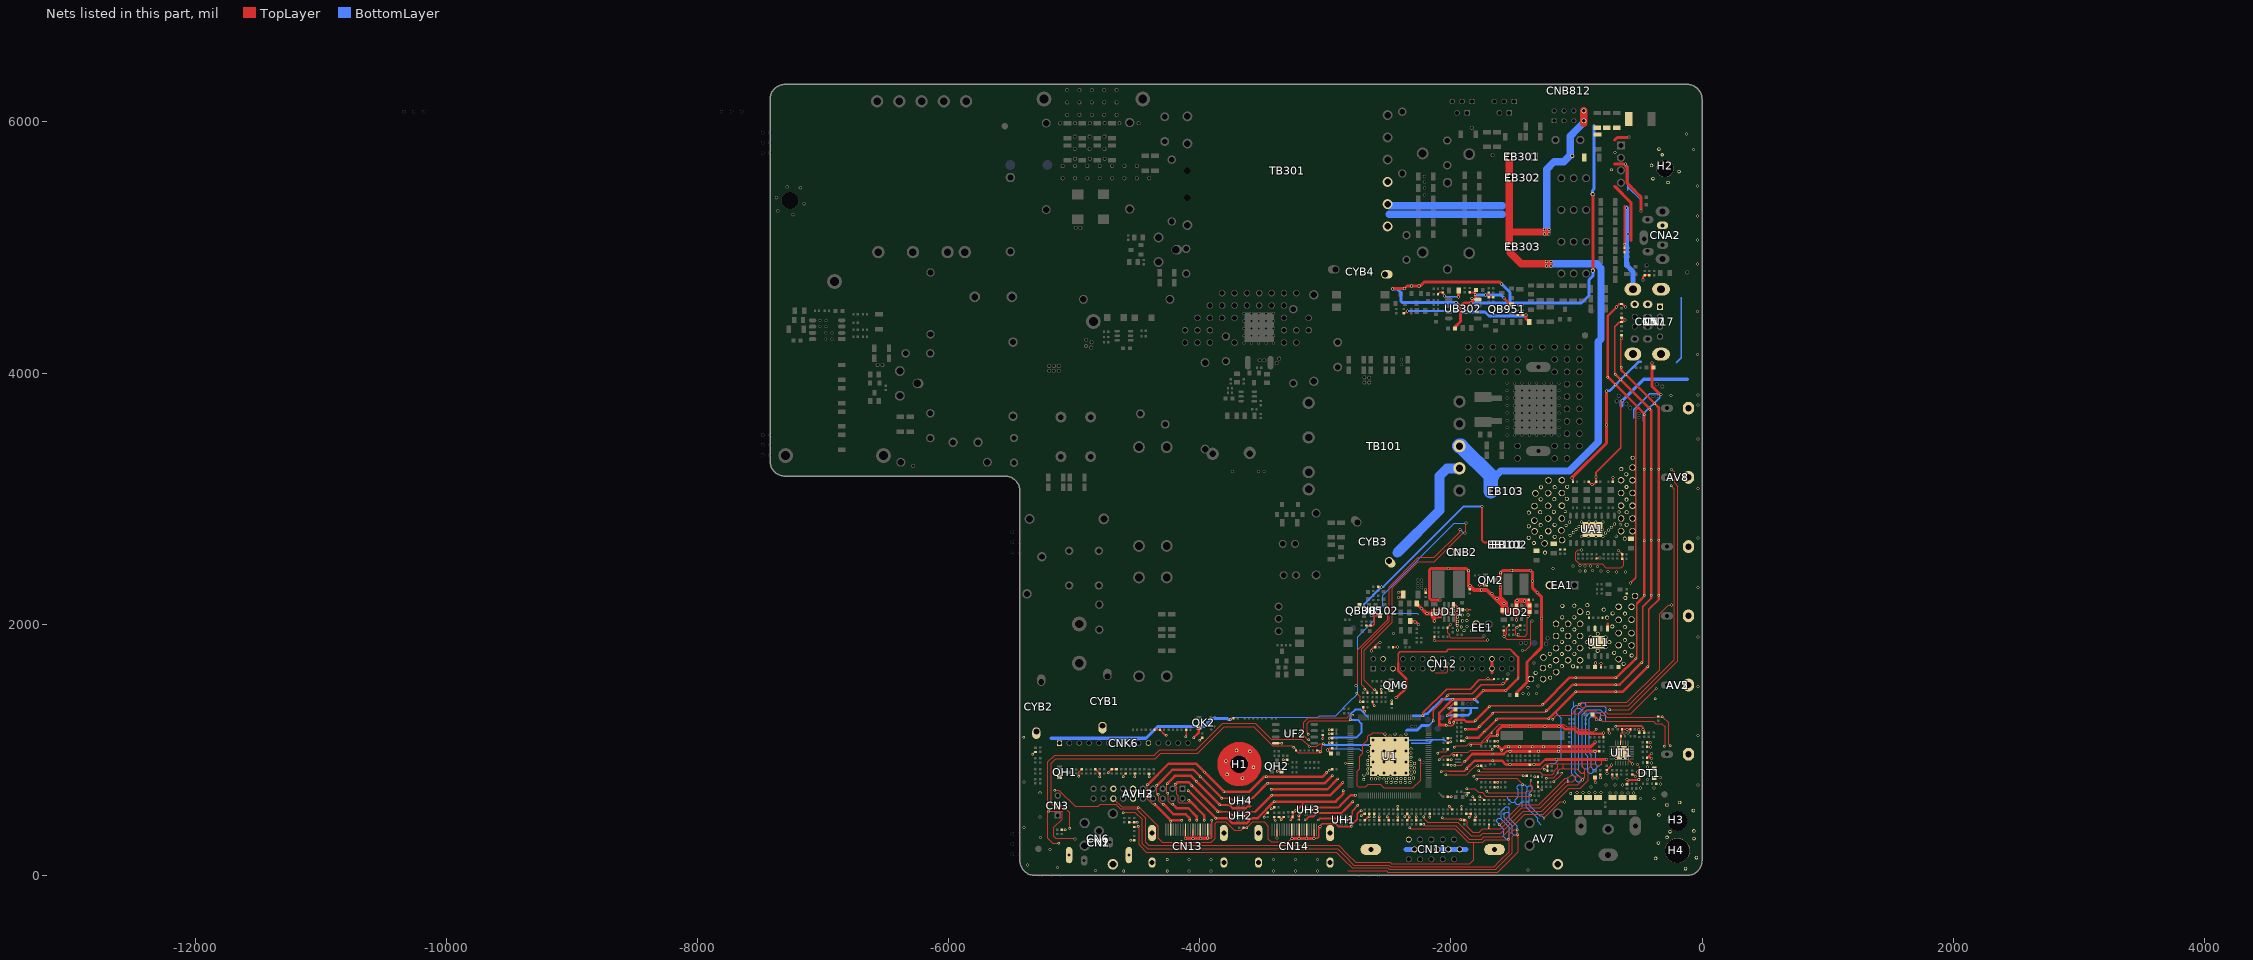
[diagram p0: the nets of this part, all layers, seen from the top]
# Altium PCB MISC84277.PcbDoc (part 8 of 15)
Units mil, origin at the board's own origin, x right, y up, seen from the top; angles counter-clockwise.
Board outline 7422.08 x 6299.21 mil, 2 copper layers (TopLayer, BottomLayer), stack 61.855 mil thick; 709 components, 395 nets, 2812 pads, 811 vias.

## Via types
v1: diameter 23.62, hole 15.75, TopLayer to BottomLayer, tented both sides, 437 vias
v2: diameter 19.68, hole 11.81, TopLayer to BottomLayer, tented both sides, 353 vias
v3: diameter 31.5, hole 23.62, TopLayer to BottomLayer, tented both sides, 16 vias
v4: diameter 31.5, hole 19.68, TopLayer to BottomLayer, tented both sides, 4 vias
v5: diameter 17.72, hole 9.84, TopLayer to BottomLayer, tented both sides, 1 vias

## Nets (pads, with @x,y where several pads share a name; then routed paths per layer and width w, separated by ;. In a path a pad name is that pad's centre, name@x,y a point inside that pad or via, vN(x,y) a via of type N, cw(c..) or ccw(c..) an arc to the next point about the centre after c; other vN are vias at no path point) (continued)
GND: AV2.2 AV2.4 AV2.6 AV5.2 AV5.4 AV5.6 AV7.1 AV8.2 AV8.4 AV8.6 AVH2.11 AVH2.12 AVH2.15 AVH2.16 AVH3.11 AVH3.12 AVH3.15 AVH3.16 C1.1 CA9.2 CA10.2 CA11.2 CA15.1 CA16.1 CA17.2 CA23.2 CA24.2 CA25.2 CA60.2 CA61.2 CB302.1 CB305.2 CB323.1 CB326.2 CB327.2 CB340.2 CB350.1 CB951.2 CD1.2 CD3.2 CD4.1 CD5.2 CD6.2 CD7.2 CD8.2 CD9.1 CD10.1 CD11.1 CD12.2 CD14.1 CD15.1 CD16.1 CD17.1 CF1.1 CF2.1 CF3.2 CF4.1 CF5.2 CF6.1 CF7.1 CF8.1 CF9.1 CF10.1 CF11.1 CF12.1 CF13.1 CF14.1 CF15.2 CF16.1 CF17.1 CF18.1 CF19.1 CF20.1 CF21.1 CF22.2 CF23.1 CF24.1 CF25.1 CF29.2 CF30.2 CF35.1 CF36.2 CF37.2 CF38.1 CF39.1 CG1.2 CG2.2 CH3.1 CH4.1 CH7.1 CH8.1 CH9.1 CH10.1 CI2.2 CI8.2 CK1.1 CK2.2 CK3.1 CK6.1 CK10.1 CL2.1 CL3.2 CL4.2 CL42.2 CL43.1 CL44.2 CM2.2 CM4.2 CM5.1 CN1.2@-4565.03,161.26 CN1.3@-5041.41,161.26 CN2.2@-4565.03,161.26 CN2.3@-5041.41,161.26 CN3.2 CN5.4 CN5.8 CN5.9 CN5.10 CN5.11 CN5.12 CN6.1 CN7.4 CN7.5 CN7.6 CN11.5 CN11.6 CN11.7 CN11.8 CN11.10 CN11.16 CN11.17 CN12.4 CN12.5 CN12.13 CN12.14 CN12.25 CN12.26 CN13.2 CN13.5 CN13.8 CN13.11 CN13.17 CN13.20 CN13.21 CN13.22 CN13.23 CN14.2 CN14.5 CN14.8 CN14.11 CN14.17 CN14.20 CN14.21 CN14.22 CN14.23 CN17.1 CNA2.1 CNB2.1 CNB812.7 CNB812.8 CNK6.1 CNK6.10 CO7.2 CO8.2 CO9.1 CO10.1 CO11.1 CT1.1 CT2.2 CT5.1 CT6.2 CT7.1 CT8.1 CT9.2 CT10.2 CT11.1 CT12.2 CT18.1 CT19.1 CT21.2 CT24.1 CT25.2 CT26.1 CT27.2 CT29.1 CT30.1 CT41.1 CT42.1 CT43.1 CT44.1 CT45.1 CT46.1 CU1.1 CV9.2 CV10.2 CYB1.1 CYB2.1 CYB3.2 CYB4.2 DB310.K DH1.A DH2.A DH3.A DH4.A DH5.A DH6.A DH7.A DH8.A DH9.A DH10.A DK1.A DT1.1 DT1.3 DU1.A DU3.A DU4.A DU7.A DU8.A EA1.2 EB101.2 EB102.2 EB103.2 EB301.2 EB302.2@-1528.48,5557.67 EB303.2@-1528.48,5005.3 EE1.2 H1.0 H1.1 H1.2 H1.3 H1.4 H1.5 H1.6 H2.0 H2.1 H2.2 H2.3 H2.4 H2.5 H2.6 H3.0 H3.1 H3.2 H3.3 H3.4 H3.5 H3.6 H4.0 H4.1 H4.2 H4.3 H4.4 H4.5 H4.6 LF6.JP_2K LT6.2 LT8.2 LT9.1 LT11.2 pad.VIA5@-534,2225 pad.VIA5@-554,2741 pad.VIA5@-554,2842.4 pad.VIA5@-554,2943.8 pad.VIA5@-554,3045.2 pad.VIA5@-554,3146.6 pad.VIA5@-554,3248 pad.VIA5@-554,3326 pad.VIA5@-562,1751 pad.VIA5@-562,1831 pad.VIA5@-562,1929 pad.VIA5@-562,2036 pad.VIA5@-562,2139 pad.VIA5@-601,2792 pad.VIA5@-601,2892 pad.VIA5@-602,2993 pad.VIA5@-602,3093 pad.VIA5@-603,3194 pad.VIA5@-611,2209 pad.VIA5@-614,2085 pad.VIA5@-615,1778 pad.VIA5@-615,1874 pad.VIA5@-615,1977 pad.VIA5@-616,2682 pad.VIA5@-625,1684 pad.VIA5@-643,3236 pad.VIA5@-645,2741 pad.VIA5@-645,2842.4 pad.VIA5@-645,2943.8 pad.VIA5@-645,3045.2 pad.VIA5@-645,3146.6 pad.VIA5@-652,2792 pad.VIA5@-660,2894 pad.VIA5@-664,1722 pad.VIA5@-664,1833 pad.VIA5@-664,1929 pad.VIA5@-664,2035 pad.VIA5@-664,2139 pad.VIA5@-684,2701 pad.VIA5@-696,2798 pad.VIA5@-701,1772 pad.VIA5@-713,2086 pad.VIA5@-715,1982 pad.VIA5@-722,2772 pad.VIA5@-738.5,1857 pad.VIA5@-746,2749 pad.VIA5@-757,2053 pad.VIA5@-770,2726 pad.VIA5@-784,2116 pad.VIA5@-831,1924.5 pad.VIA5@-831.5,1788.5 pad.VIA5@-870.08,4816.93 pad.VIA5@-872.05,5425.2 pad.VIA5@-910,2089 pad.VIA5@-913.39,2151.57 pad.VIA5@-914.5,1857.5 pad.VIA5@-971.5,1713.07 pad.VIA5@-971.5,1809.72 pad.VIA5@-971.5,1906.36 pad.VIA5@-971.5,2003 pad.VIA5@-971.5,2099.64 pad.VIA5@-979,2778 pad.VIA5@-1003,2755 pad.VIA5@-1017,1764 pad.VIA5@-1017,1858 pad.VIA5@-1017,1958 pad.VIA5@-1017,2054.64 pad.VIA5@-1017.72,2147.64 pad.VIA5@-1026,2732 pad.VIA5@-1028,1665 pad.VIA5@-1033.45,5730.08 pad.VIA5@-1051,2708 pad.VIA5@-1054.5,2812.85 pad.VIA5@-1067.25,1713.07 pad.VIA5@-1067.25,1809.72 pad.VIA5@-1067.25,1906.36 pad.VIA5@-1067.25,2003 pad.VIA5@-1075,3094 pad.VIA5@-1077,2999 pad.VIA5@-1082,2786 pad.VIA5@-1090,2896 pad.VIA5@-1112.2,2145.67 pad.VIA5@-1114,1958 pad.VIA5@-1114,2054.64 pad.VIA5@-1115,2670 pad.VIA5@-1116,1667 pad.VIA5@-1116,1763 pad.VIA5@-1116,1859 pad.VIA5@-1117,2842.4 pad.VIA5@-1117,2943.8 pad.VIA5@-1117,3045.2 pad.VIA5@-1117,3146.6 pad.VIA5@-1121,2747 pad.VIA5@-1162,1619 pad.VIA5@-1163,1713.07 pad.VIA5@-1163,1809.72 pad.VIA5@-1163,1906.36 pad.VIA5@-1163,2003 pad.VIA5@-1174,3092 pad.VIA5@-1175,2696 pad.VIA5@-1175,2791 pad.VIA5@-1177,2996 pad.VIA5@-1181,2894 pad.VIA5@-1204.72,4852.36 pad.VIA5@-1204.72,4887.8 pad.VIA5@-1210,1574 pad.VIA5@-1211,1667 pad.VIA5@-1213,1764 pad.VIA5@-1220.47,5108.27 pad.VIA5@-1220.47,5143.7 pad.VIA5@-1223.2,3145.2 pad.VIA5@-1225,2741 pad.VIA5@-1226,2841 pad.VIA5@-1226,2942.4 pad.VIA5@-1226,3043.8 pad.VIA5@-1240.16,4852.36 pad.VIA5@-1240.16,4887.8 pad.VIA5@-1251,2571 pad.VIA5@-1254,2644 pad.VIA5@-1255.91,5108.27 pad.VIA5@-1255.91,5143.7 pad.VIA5@-1264,1736 pad.VIA5@-1266,1563 pad.VIA5@-1267,1651 pad.VIA5@-1282,2694 pad.VIA5@-1283,3090.6 pad.VIA5@-1286,2790 pad.VIA5@-1286,2994.6 pad.VIA5@-1290,2892.6 pad.VIA5@-1326,1612 pad.VIA5@-1327.5,3042.5 pad.VIA5@-1334,2740 pad.VIA5@-1335,2941 pad.VIA5@-1336,2825 pad.VIA5@-1339,2647 pad.VIA5@-1363,1564 pad.VIA5@-1379.3,2889 pad.VIA5@-1380,2780 pad.VIA5@-1381,2687 pad.VIA5@-1596,4709 pad.VIA5@-1832.68,4592.52 pad.VIA5@-1836.61,1948.82 pad.VIA5@-1863,2074 pad.VIA5@-1874,2030 pad.VIA5@-1879.92,4487.1 pad.VIA5@-1895.67,1948.82 pad.VIA5@-1910,2027 pad.VIA5@-1912,2074 pad.VIA5@-1923,4495.5 pad.VIA5@-1929.13,4535.43 pad.VIA5@-1948,2022 pad.VIA5@-1948,2058 pad.VIA5@-1948.82,1952.76 pad.VIA5@-1950,1991 pad.VIA5@-1958.5,4561.5 pad.VIA5@-1980,2109 pad.VIA5@-2002,2087 pad.VIA5@-2030,2110 pad.VIA5@-2087.7,2097.06 pad.VIA5@-2253.94,4693.81 pad.VIA5@-2290.9,823 pad.VIA5@-2290.9,856.8 pad.VIA5@-2290.9,890.6 pad.VIA5@-2297.6,775.2 pad.VIA5@-2314.96,4693.81 pad.VIA5@-2319.2,805.4 pad.VIA5@-2319.2,839.2 pad.VIA5@-2319.2,873 pad.VIA5@-2319.2,906.8 pad.VIA5@-2319.2,940.6 pad.VIA5@-2319.2,974.4 pad.VIA5@-2319.2,1008.2 pad.VIA5@-2327.2,741 pad.VIA5@-2330.3,770.9 pad.VIA5@-2358.3,1124.32 pad.VIA5@-2364.1,770.9 pad.VIA5@-2364.4,741 pad.VIA5@-2370.87,4674 pad.VIA5@-2397.9,770.9 pad.VIA5@-2401.6,741 pad.VIA5@-2431.7,770.9 pad.VIA5@-2438.8,741 pad.VIA5@-2445,1124 pad.VIA5@-2465.5,769.2 pad.VIA5@-2466.54,4671.26 pad.VIA5@-2476,741 pad.VIA5@-2499.3,769.2 pad.VIA5@-2513.2,741 pad.VIA5@-2525.21,1124.32 pad.VIA5@-2533.1,769.2 pad.VIA5@-2566.9,769.2 pad.VIA5@-2600.7,769.2 pad.VIA5@-2634.5,769.2 pad.VIA5@-2635.5,864.3 pad.VIA5@-2648.2,948.3 pad.VIA5@-2662.7,814 pad.VIA5@-2662.7,847.8 pad.VIA5@-2662.7,881.6 pad.VIA5@-2662.7,915.4 pad.VIA5@-2693.4,797.4 pad.VIA5@-2694.55,765.25 QB305.E QB951.E QH1.E QH2.E QK2.E QM2.E QM6.E RA1.1 RA7.JP_2K RA9.1 RA11.JP_2K RA14.1 RB134.2 RB337.1 RB338.1 RB339.1 RB340.1 RB341.1 RB345.2 RB352.2 RB355.2 RB357.1 RB364.1 RB385.1 RB951.1 RD7.1 RD16.1 RF12.2 RF13.2 RF14.1 RF15.1 RF16.2 RF18.2 RF19.2 RH55.2 RI5.1 RI7.2 RI9.1 RI11.2 RI13.1 RI15.1 RI17.1 RI18.1 RM6.2 RM10.2 RO3.1 RO7.1 RO10.2 RO12.2 RV2.1 RV4.1 RV5.1 RV8.2 RV11.1 RV13.2 RV14.2 TB101.8@-1932.31,3241.33 TB101.9@-1932.31,3418.5 TB301.1 TB301.2@-2504.74,5345.75 TB301.3@-2504.74,5522.92 U1.116 U1.129 UA1.EPAD@-874.02,2754.94 UB102.A UB302.4 UD2.2 UD11.1 UF2.4 UH1.GND UH2.GND UH3.GND UH4.GND UL1.1 UL1.3 UL1.EPAD UT1.10 UT1.25 | length 142392
  TopLayer w4: v2(-5203.6,509.3) -5202.69,510.21 -5100.22,510.21 -5096.94,506.94 ; -3575,1210.16 -3558.36,1210.16 -3431.01,1082.81 -3334.78,1082.81
  TopLayer w5: v2(-4417.02,720.92) -4418.8,719.13 -4418.8,609.76 -4376.84,567.8 v2(-4359.93,567.8) ; v2(-4342.78,716.45) -4341.54,715.21 -4341.54,641.89 -4328.4,628.76 -4328.4,594.96 -4301.22,567.78 ; v2(-4260.82,729.12) -4262.3,727.64 -4262.3,659.1 -4249.9,646.7 -4249.9,590.49 -4226.31,566.9 v2(-4215.7,566.9) ; CN13.17@-4232.29,364.62 -4232.29,429.51 v2(-4232.1,429.7) ; v2(-4195.46,725.18) -4195.46,714.57 -4184.06,703.16 -4184.06,645.06 -4171.7,632.7 -4171.7,587 -4162.1,577.4 -4075.03,577.4 -4069.75,582.67 ; -3065.26,1031.19 -3064.24,1031.19 -3057.09,1038.34 ; UT1.25@-639.4,975.31 -574.17,910.09
  TopLayer w6: AVH2.16@-4689,610.96 -4623.14,545.1 -4518,545.1 ; v2(-4490.6,538) -4497.7,545.1 -4518,545.1 ; v2(-4146.1,273.5) -4136.1,263.5 -4127.4,263.5 ; CH10.1@-3652.97,378.1 -3670.81,360.26 -3727.16,360.26 -3792.95,426.05 -3866.44,426.05 -3877,415.5 -3877,294.47 -3907.97,263.5 -4127.4,263.5 ; v2@-3628.2,378.1 -3624.56,378.1 -3576.61,426.05 -3488.61,426.05 -3453.5,390.94 -3453.5,286.94 -3432.25,265.69 -3297.25,265.69 v1@-3267.72,295.22 ; v2(-3137,1123) -3137,1129 -3146,1138 -3146,1211.56 -3124.56,1233 -2809,1233 v2(-2801,1241) ; v2(-3132,1080) -3141,1080 -3172,1111 -3172,1219 -3136,1255 -2893,1255 ; -2880,1255 -2893,1255 ; -2852.31,123.69 -2787.68,59.06 -2503.83,59.06 -2493.14,48.38 -1642.35,48.38 -1599.23,91.5 ; -2847.42,155.58 -2772.91,81.06 -2494.72,81.06 -2484.03,70.38 -1657.12,70.38 -1610,117.5 ; v2(-2839.93,893.65) -2837.83,891.56 U1.116@-2800.46,891.56 ; -2824.54,169.46 -2760.14,105.06 -2484.77,105.06 -2474.09,94.38 -1849.62,94.38 -1818.35,125.65 -1818.35,180.15 ; v2(-2783,1277) -2790.16,1269.84 -2812.95,1269.84 -2827.79,1255 -2893,1255 ; v1(-2755.9,1513.78) -2751.97,1513.78 -2741,1524.75 -2741,1549.21 ; -2741,1553.15 -2741,1549.21 ; -2712.27,1776 -2712.27,1802.96 ; CG1.2@-2665.27,1454 -2665.27,1469.27 -2712.27,1516.27 -2712.27,1802.96 ; -2664.14,718.86 -2659.26,723.74 ; -2661.98,1087.8 -2661.98,1081.2 ; -2641.3,1119.5 -2650.57,1119.5 ; v3(-2620.6,1077.82) U1.129@-2489.44,946.68 -2489.44,1075.87 -2547.57,1134 -2550.4,1134 ; v2@-2613.58,1478.58 -2690.27,1555.27 -2690.27,1793.84 -2468,2016.11 -2468,2291.37 -2260.37,2499 -2133.27,2499 -1905.9,2726.37 v1(-1889.76,2726.37) -1881.89,2734.24 v1(-1881.89,2807.09) ; v2(-2606,1480) -2600,1480 -2591.27,1471.27 CG2.2@-2591.27,1454 ; CG2.2@-2593,1454 CG2.2@-2591.27,1454 ; CG2.2@-2591.27,1456.27 CG2.2@-2591.27,1454 ; -2571,1134 -2550.4,1134 ; v2@-2522,2084 -2521,2085 -2506.26,2085 -2501.97,2080.71 -2501.97,2034.86 -2741,1795.83 -2741,1549.21 ; v2(-2248.34,920.93) -2241.5,914.09 -2241.5,888.5 ; -2241.5,902.3 -2241.5,888.5 ; v2(-2105,973) v2@-2105,972.89 ; v2@-2100.11,968 v2@-2105,972.89 ; v2@-2092.05,922 v2(-2093,922) -2062,953 -2009,953 -1982,980 -1861.04,980 -1843.54,997.5 -1676.57,997.5 v2(-1669.72,1004.34) ; CF20.1@-2025,1006 -2025,1000 -2039,986 -2091.89,986 v2@-2105,972.89 ; v2(-1972,1022) -1963.5,1030.5 -1876.19,1030.5 -1850.19,1056.5 -1763.71,1056.5 -1691.41,1128.81 ; v1(-1929.13,2755.91) -1929.13,2734.25 -2131.89,2531.49 -2258.99,2531.49 -2490,2300.48 -2490,2236.22 -2490,2025.23 -2712.27,1802.96 ; v2(-1844.2,1037.4) -1836.96,1044.64 -1759.91,1044.64 -1740.86,1063.7 ; v2(-1713.1,1066.9) -1716.3,1063.7 -1740.86,1063.7 ; v2(-1673.1,1134.8) -1673.1,1147.11 ; -1668.6,1151.61 -1668.6,1139.3 -1679.09,1128.81 -1691.41,1128.81 ; v2(-1630,1114) -1674,1114 -1724.3,1063.7 -1740.86,1063.7 ; v2(-841.4,1163.9) -861.11,1144.19 -891.39,1144.19 -911.4,1164.2 -991.09,1164.2 -1008.99,1182.1 -1077.06,1182.1 -1100.01,1205.06 -1615.15,1205.06 -1691.41,1128.81 ; -4518,545.1 -4487.93,545.1 -4332.1,389.27 -4332.1,295.57 -4299.33,262.8 -4128.1,262.8 -4127.4,263.5 ; -2661.98,1081.2 -2702.06,1041.12 -2702.06,973.5 -2726.84,948.71 -2726.84,848.75 -2745.5,830.09 -2745.5,710.4 -2739.1,704 -2679,704 -2659.26,723.74 ; -2661.98,1081.2 -2661.98,1108.09 -2650.57,1119.5 ; -2659.26,723.74 -2561.54,723.74 -2533.63,695.83 -2304.46,695.83 -2241.5,758.78 -2241.5,888.5 ; -2650.57,1119.5 -2637.56,1119.5 -2623.06,1134 -2550.4,1134
  TopLayer w7: v1(-2131.89,1872.04) -2131.73,1872.2 RD16.1@-2131.73,1900 v1@-2131.73,1877.8 ; v2(-2078.9,827) -2076.59,824.7 v2@-2076.59,824.3 ; v2@-2078.86,829.69 -2075.31,833.24 -2017.24,833.24 -2014,830 ; v2(-2042.7,802.9) -2041.6,801.8 -1874.6,801.8 -1837.1,839.3
  TopLayer w8: v2(-5332,963.8) -5312.9,982.9 DK1.A@-5308.96,982.9 ; -5209.5,316.2 -5209.5,570.4 ; v2(-5157,679.4) -5122.8,679.4 -4993.36,549.96 -4807.52,549.96 -4791.99,565.5 -4667.9,565.5 -4632.9,530.5 -4506,530.5 -4431.5,456 -4431.5,263.7 -4406.3,238.5 -4257.2,238.5 ; v2(-5123.3,256.5) -5171.2,256.5 -5209.5,294.8 -5209.5,570.4 ; v2@-5116.3,812.98 v2(-5115.1,814.18) ; CO7.2@-5098.6,363.53 -5073.27,363.53 v2(-5072.9,363.9) ; -5096.94,506.94 -5096.94,448.3 -5162.4,382.84 -5162.4,309.9 -5146.7,294.2 -5000.2,294.2 v1(-4994.9,288.9) ; v2(-5035.9,376.9) -5035.9,496.9 -5095.36,556.36 CN3.2@-5131.53,556.36 -5165.26,556.36 -5183.5,574.6 -5183.5,892.55 -5146.2,929.84 -4353.23,929.84 -4309.87,973.2 -4017.27,973.2 -3806.32,1184.16 -3571.95,1184.16 -3418.4,1030.6 -3262.9,1030.6 v2(-3253.8,1021.5) v2@-3260.22,1021.5 ; v2(-4609.1,498.6) -4603.2,504.5 -4516.77,504.5 -4457.5,445.23 -4457.5,296.2 ; RO7.1@-4563.06,422.97 -4497.67,422.97 v2(-4497.2,422.5) ; v2(-4548.6,279.5) -4548.27,279.17 CO11.1@-4522.9,279.17 ; RO3.1@-4522.89,386.23 -4494.67,386.23 v2(-4489.4,391.5) -4483.5,385.6 -4483.5,242.16 -4425.84,184.5 -2913.12,184.5 -2852.31,123.69 ; -4457.5,317.2 -4457.5,296.2 ; -4301.5,210.5 -4290.8,210.5 ; -4269.5,238.5 -4257.2,238.5 ; v1@-4114.18,306.8 -4113.79,306.41 -3910.19,306.41 -3900,316.6 ; v1@-3936.33,295.18 -3908.82,295.18 -3900,304 -3900,316.6 ; -3910.46,303.07 -3903.21,310.32 -3903.21,423.89 -3900,427.1 -3900,392.9 ; v2@-3906.6,443 -3900,436.4 -3900,392.9 ; -3561.18,1210.16 -3817.09,1210.16 -4028.04,999.2 -4320.64,999.2 -4364,955.84 -5156.97,955.84 -5209.5,903.32 -5209.5,570.4 ; -3365.58,1084.81 -3186.51,1084.81 -3127.97,1026.27 -3070.18,1026.27 -3065.26,1031.19 ; RO10.2@-3234.13,994.42 -3215.15,975.44 -3035.38,975.44 -3029.91,980.92 -3029.91,1027.42 -3017.7,1039.63 v2(-3017.7,1048) -3045.31,1048 -3053.47,1039.84 ; CO8.2@-3064.27,994.42 -3050.92,994.42 -3041.5,985 v2(-3039.5,985) ; -2847.42,155.58 -2902.35,210.5 -4290.8,210.5 ; -2824.54,169.46 -2893.58,238.5 -4257.2,238.5 ; -2821.96,36.06 -2513.35,36.06 -2501.79,24.5 -1628.6,24.5 -1466,187.1 -1466,261 ; v2(-2751,1449) -2724,1422 v2(-2724,1381) ; RM10.2@-2520.27,1545 -2489,1513.73 v2(-2489,1510) ; RF16.2@-2423,524.73 v2(-2423,552) ; v2@-2326,377 v2(-2327,378) -2319,370 -1970.77,370 -1863.82,263.06 -1817.5,263.06 ; RI13.1@-2242,406.27 -2216.27,406.27 v2(-2216,406) -2206,396 -1960,396 -1853.06,289.06 -1756.09,289.06 -1737.15,308 -1592.23,308 -1414.23,486 -1266.88,486 -1059.12,693.76 -970.18,693.76 -908.31,755.63 -908.31,850.88 -870.21,888.98 ; v2(-2218,465) -2218,454.38 -2185.62,422 -1944.18,422 -1837.24,315.06 -1766.86,315.06 -1747.92,334 -1603,334 -1425,512 -1277.65,512 -1069.89,719.76 -992,719.76 v1(-953,758.76) ; v1@-2131.73,1877.8 -2121.74,1867.8 -1716.03,1867.8 -1709.65,1874.18 v1(-1709.65,1875.61) ; -2127,1614.1 -2038,1614.1 -2025.48,1626.62 v1@-2025.48,1683.19 ; v2(-2071,457) -2065,451 -1890,451 -1871,432 -1871,385.59 -1827.47,342.06 -1810,342.06 ; CD7.2@-2027.27,1972 -2027.27,1932.78 -2009.41,1914.92 -2009.41,1900.53 -2002.68,1893.8 -1745.96,1893.8 -1738.19,1901.58 v1(-1738.19,1907.48) ; CF14.1@-2025,881 -2002,881 v2(-1999,878) ; v2(-1969.2,878) -1919.2,878 v2(-1889.11,908.09) ; v2(-1920.68,443.53) -1916.88,439.73 RI17.1@-1895,439.73 ; RF12.2@-1916,523.73 v2(-1916,549) ; v2(-1874.1,691.2) -1809.2,691.2 -1779,661 -1752,661 -1722.84,631.84 -1370.16,631.84 v2(-1364,638) ; v2(-1873,637) -1871,637 -1862.4,645.6 LF6.JP_2K@-1862.4,658.4 ; -1837.1,839.3 -1802.4,874 v2(-1787,874) ; -1826.06,342.06 -1810,342.06 ; v2(-1820.4,791) -1811.4,800 -1431.35,800 v2(-1425.43,794.08) -1397.81,794.08 CF29.2@-1396.73,793 ; -1818.35,180.15 -1818.35,262.2 -1817.5,263.06 ; v2(-1793.6,764.4) -1784,774 -1477,774 -1429,726 v2(-1429,722) ; v2@-1784,874 CT19.1@-1758.73,874 -1764,874 -1740,850 -1281,850 -1242.02,888.98 -899.5,888.98 ; v2(-1780.4,834) -1771.4,825 -1292,825 -1270,803 -1193,803 -1178,818 -1178,835.01 -1151.01,862 -1151.01,888.98 ; v2@-1774.54,622.92 -1757.08,622.92 -1735,600.85 RI7.2@-1735,600.73 ; v2@-1773.32,627.32 v2(-1770.68,627.32) ; v2(-1716,671) -1701.84,656.84 -1399.16,656.84 -1382.49,673.51 -1362.49,673.51 -1351,685 -1351,708.73 -1363.27,721 v5(-1363.27,757) ; RV4.1@-1653.27,701 v2(-1628,701) ; v2(-1616,404) -1607.74,404 -1447.74,564 -1299.19,564 -1091.43,771.76 -1070.24,771.76 -1042.74,799.26 -1028.2,799.26 -1012,783.06 ; -1610,117.5 -1537.69,189.81 -1537.69,325.77 -1500.46,363 v2@-1472,363 ; -1599.23,91.5 -1511.69,179.04 -1511.69,307.31 -1496.84,322.16 -1483.2,322.16 ; -1591,282 -1624,282 ; v1(-1577,1901) -1556,1880 -1370,1880 ; -1561.53,884.53 v1@-1523.24,884.53 ; v2(-1543.53,287.79) -1549.32,282 -1624,282 ; v1@-1484,1975 -1484,1918 -1472,1906 -1409.38,1906 -1393,1922.38 -1393,2053 v1(-1386,2060) ; v1(-1474.4,1975.89) -1474.4,1976.6 -1461,1990 CD17.1@-1447.73,1990 ; v2(-1471,364) v2@-1472,363 ; v2(-1467,322) -1467.16,322.16 -1483.2,322.16 ; -1466,294.5 -1466,261 ; v1(-1431,1791) -1404,1791 -1364,1831 -1364,2021 -1358.75,2026.25 v1(-1355.7,2026.25) ; v2(-1334,787) -1331,784 RF14.1@-1307.73,784 ; RI9.1@-1307.73,743 RI11.2@-1307.73,707 -1281.73,681 v2(-1275,681) ; v2(-1259,454) -1259,457.12 -1131.12,585 v1(-1097,585) ; v2(-1257,845) -1256,846 -1256,847 -1243.73,847 CF30.2@-1230.73,834 RF15.1@-1230.73,870 ; v2(-1240.57,772.16) -1234.72,778 -1182.64,778 -1153,807.64 -1153,824.66 -1128.66,849 -1111.64,849 -1106.5,854.15 -1106.5,858.07 ; v2(-1189.7,1244.9) -1160.1,1274.5 ; v2@-1187,1247.6 -1160.1,1274.5 ; v2@-1179.44,744.44 -1117.54,806.34 v2(-1117.54,815.09) ; -1106.5,886.47 -1106.5,858.07 ; v1@-960,758.76 v1(-953,758.76) ; v1(-959,2591.5) -986,2591.5 -1005.84,2571.66 -1005.84,2509.34 -976.41,2479.91 -795.02,2479.91 -766.3,2451.19 -644.81,2451.19 -624.51,2471.49 -624.51,2510.76 CA9.2@-635.73,2521.99 ; -950.43,887.41 -950.43,859.55 -934.31,843.43 ; -934.31,807 -941.26,813.95 -946.88,813.95 ; -868.15,888.98 -899.5,888.98 ; v1@-844.65,1239.65 v1@-843,1238 ; -809.76,1266.8 -814.1,1262.45 -814.1,1243.98 -809.76,1239.64 v2(-810.8,1238.6) -799.46,1227.26 -390.26,1227.26 -371,1208 -321,1208 -295,1182 -295,1035 v2(-301,1029) ; -809.76,1266.84 -802.8,1273.8 -775.5,1273.8 -759.57,1257.87 -379.92,1257.87 -373.06,1264.73 CI8.2@-348,1264.73 v2(-317.73,1264.73) -266.53,1213.53 -266.53,1044.53 v2(-253,1031) ; -798,922.98 -798,893.83 -819.38,872.45 -836.62,872.45 -853.15,888.98 -899.5,888.98 ; v2(-734.1,1317.3) -584.93,1317.3 -192.32,1709.92 -192.32,1955 ; v2(-364.17,1488.19) -566.93,1285.43 -750.36,1285.43 -764.73,1299.8 -839.3,1299.8 -849.46,1309.96 -951.31,1309.96 -973.16,1288.11 -1014.91,1288.11 -1022.5,1295.7 ; v2(-247.4,3102.3) -220.32,3075.22 -220.32,1718.68 -588.16,1350.84 -922.51,1350.84 -937.4,1335.96 -954.6,1335.96 -979.4,1360.76 v2(-979.4,1361.44) ; v1(-245.5,2152) -270.04,2152 -338.74,2083.3 -338.74,1637.03 -598.93,1376.84 -964,1376.84 v2(-979.4,1361.44) ; v1(-244.5,3234) -219,3208.5 -219,3127.15 -192.32,3100.46 -192.32,1955 ; -192.32,1932.6 -192.32,1955 ; -4457.5,296.2 -4457.5,252.93 -4415.07,210.5 -4290.8,210.5 ; -3900,316.6 -3900,392.9 ; -1817.5,263.06 -1745.32,263.06 -1726.38,282 -1624,282 ; -1810,342.06 -1776.63,342.06 -1746.69,372 -1602.97,372 -1436.97,538 -1288.42,538 -1080.66,745.76 -1031.24,745.76 -1012,765 -1012,783.06 ; -1483.2,322.16 -1472,333.35 v2@-1472,363 ; -1483.2,322.16 -1466,304.96 -1466,261 ; -1160.1,1274.5 -1043.7,1274.5 -1022.5,1295.7 ; -1106.5,858.07 -1097.42,849 -999.17,849 -964.12,813.95 -946.88,813.95 ; -1022.5,1295.7 -1022.5,1305.9 -990.6,1337.8 -990.6,1350.25 v2(-979.4,1361.44) ; -1012,783.06 -1002.06,793 -985.17,793 -964.12,771.95 -946.88,771.95 -934.31,784.52 -934.31,792.76 ; v1(-953,758.76) -934.31,777.45 -934.31,792.76 ; -946.88,813.95 -934.69,826.14 -934.69,843.05 -934.31,843.43 ; -934.31,792.76 -934.31,843.43
  TopLayer w10: v1(-4114.18,295.18) CN13.11@-4114.18,364.62 ; v1(-4055.12,295.18) CN13.8@-4055.12,364.62 ; v1(-3996.07,295.18) CN13.5@-3996.07,364.62 ; v1@-3937.01,295.18 CN13.2@-3937.01,364.62 v1(-3937.01,295.85) ; -3835.1,508.05 -3771.72,508.05 -3736.83,473.17 UH2.GND@-3695.54,473.17 ; v2(-3823.95,614.05) -3756.09,614.05 -3734.36,592.32 UH4.GND@-3654.6,592.32 -3652.7,594.22 -3609.38,594.22 -3594.8,608.8 ; v2(-3730.9,481.6) -3722.47,473.17 UH2.GND@-3695.54,473.17 ; v2@-3727.17,473.17 UH2.GND@-3695.54,473.17 ; v2(-3606.6,608.8) -3594.8,608.8 ; -3589.54,614.05 -3594.8,608.8 ; -3556.95,508.05 -3597.85,508.05 -3632.73,473.17 UH2.GND@-3695.54,473.17 ; CN14.17@-3385.83,364.62 -3385.83,296.83 v1(-3385.5,296.5) ; DH7.A@-3370,465.27 -3351.5,446.77 v2(-3351.5,441.5) -3351.5,445.77 DH6.A@-3332,465.27 ; CN14.11@-3267.72,364.62 -3267.72,295.22 v1(-3267.5,295) -3064,295 -3052,307 -3052,367.44 ; CH7.1@-3261.17,466.4 -3276.9,450.67 v2(-3276.9,441) -3257.24,460.66 -3257.24,499.44 DH10.A@-3261.5,503.7 -3243.36,503.7 v2@-3236.8,510.26 ; v2(-3236.8,517.11) v2@-3236.8,510.26 ; -3222.26,524.8 -3216.18,530.88 ; v2(-3213.4,440.8) -3210.02,444.18 -3210.02,477.64 -3196.58,491.08 ; v2(-3211.18,473.87) -3211.18,476.48 -3196.58,491.08 ; CN14.8@-3208.66,364.62 -3208.66,295.22 v1(-3208.44,295) ; -3174.4,587.84 -3180.39,581.84 -3180.39,566.66 -3216.18,530.88 ; v2(-3162.5,441.1) -3161.6,440.2 -3156.48,440.2 -3131.15,465.53 -3097.89,465.53 -3066.08,497.34 -3038.6,497.34 ; CN14.5@-3149.61,364.62 -3149.61,295.22 v1(-3149.39,295) ; CN14.2@-3090.55,364.62 -3090.55,295.22 v1(-3090.33,295) ; -3064.5,541.34 -3077.24,541.34 -3097.47,521.1 UH3.GND@-3113.7,521.1 -3166.56,521.1 -3196.58,491.08 ; v1@-3046,396.84 -3052,390.84 -3052,378 ; v1@-3036.25,383.19 -3052,367.44 ; -2912.7,453.34 -2904.16,453.34 -2892.13,441.3 UH1.GND@-2835.03,441.3 -2813.7,441.3 v2(-2803.4,451.6) -2786.2,468.8 -2786.2,511.96 v2(-2741.66,556.5) ; -2828.9,387.8 -2873.4,387.8 ; v2(-2794.2,391.9) -2794.2,398.8 -2786.4,406.6 ; v2(-2724,1381) RF18.2@-2698.73,1381 ; v2(-2714.8,514.4) -2721.76,514.4 -2734.93,501.23 ; v2@-2713.23,522.93 -2734.93,501.23 ; -2698.73,1323.73 CF17.1@-2698.73,1337 -2698.73,1318.73 -2688,1308 v2(-2686,1308) ; RV14.2@-2685,438.73 -2685,439.62 -2659.62,465 v2(-2650,465) -2649,466 CV10.2@-2649,491.27 ; RF13.2@-2624.73,1381 -2624.73,1365.73 -2610,1351 v2(-2609.16,1351) ; v2(-2610,466) CV9.2@-2610,491.27 ; -2421.15,1688.46 -2421.15,1765.85 -2406,1781 -2037.9,1781 -2020.1,1798.8 -1978,1798.8 ; v2(-2225,1272) -2225,1294 -2035,1484 -1848.16,1484 -1774.25,1557.9 -1662.26,1557.9 CF36.2@-1656.34,1563.82 ; v2(-2142.8,1232.8) -2142.8,1314.2 -2012,1445 ; CD5.2@-2132.7,2081.32 -2152.89,2101.51 ; -2098.5,1221 -2098.5,1197 -2092.5,1191 -1993.29,1191 -1979,1205.29 v2(-1979,1220) ; v2(-2027.85,1429.15) -2012,1445 ; CF19.1@-2025.27,1092 -2002,1092 v2(-2000,1094) ; CF24.1@-2025,1056 -2008,1056 -2000.3,1063.7 v2(-2000.3,1063.93) ; -2016.92,1798.8 -1978,1798.8 ; v2(-2015.2,549) -2013.27,549 CI2.2@-1988,523.73 ; -1991.7,2165.85 -1991.7,2125.85 -1997.71,2119.84 -2044.5,2119.84 -2050.5,2113.85 -2152.44,2113.85 -2152.89,2113.39 -2152.89,2101.51 ; -1960.24,2076.38 -1961.7,2077.85 -1969.5,2077.85 ; pad.VIA5@-1946.4,1980.4 -1958.48,1992.48 -1958.48,2070.99 -1965.33,2077.85 -1969.5,2077.85 ; CO9.1@-1880,490.27 RO12.2@-1844,490.27 -1844,475 v2(-1856,463) ; v2(-1828,626) -1828,625 -1809,606 RI5.1@-1809,600.73 ; v2(-1697,380) RI18.1@-1697,405.27 ; CF35.1@-1552.01,1563.82 -1552.01,1555.99 -1589.1,1518.9 -1758.1,1518.9 -1832,1445 -2012,1445 ; -1500,1771 -1527.8,1798.8 -1978,1798.8 ; UT1.10@-649.76,1056.02 -649.76,1112.68 -649.76,1117.57 ; -574.17,910.09 v1(-552.52,888.43) ; v1(-569,2329) -526.5,2371.5 -526.5,3702.95 -505.58,3723.86 ; v2@-3236.8,510.26 -3216.18,530.88 ; -3052,367.44 -3052,378 ; -3052,378 -3052,384.83 -3025,411.84 -2919.04,411.84 -2895,387.8 -2873.4,387.8 ; -2873.4,387.8 -2805.2,387.8 -2786.4,406.6 ; -2786.4,406.6 -2745.4,447.6 -2745.4,490.76 -2734.93,501.23 ; -2152.89,2101.51 -2152.14,2100.75 -2152.14,2057.07 -2147.31,2052.25 -2101.15,2052.25 -2097.77,2055.63 -2080.93,2055.63 -2076.93,2059.62 -2076.93,2073.62 -2072.7,2077.85 -1969.5,2077.85
  TopLayer w11: v2@-697,3990.23 -697,4368 -658.77,4406.23 DU8.A@-641.5,4406.23 ; -649,4028.5 -649,4169.5 ; -649,4181 -649,4169.5 ; DU7.A@-641.5,4301.77 -641.5,4275 -649,4267.5 -649,4169.5 ; v2@-531.55,1724.24 -519.24,1736.54 -519.24,1958 ; -519.24,1940.13 -519.24,1958 ; v2@-477.59,1697.59 -471.24,1703.93 -471.24,1981 ; -471.24,1947.83 -471.24,1981 ; -471,2206.31 -519.24,2158.07 -519.24,1958 ; -423.24,1664.96 -423.24,2118.3 -342.5,2199.04 -342.5,2253.5 ; -403.5,2205.92 -471.24,2138.18 -471.24,1981 ; DU8.A@-641.5,4406.23 DU3.A@-641.5,4441.27 -630.27,4441.27 v1(-613.5,4424.5) -631.77,4406.23 DU8.A@-641.5,4406.23